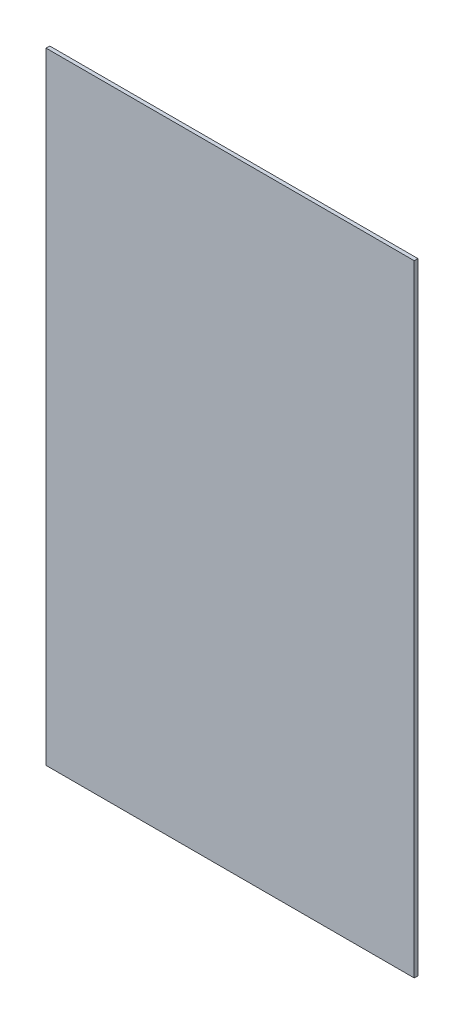
SolidWorks part; units mm, degrees
material "PMMA(有机玻璃)"
ref_plane "前视" through (0, 0, 0) normal (0, 0, 1) x (1, 0, 0)
ref_plane "上视" through (0, 0, 0) normal (0, 1, 0) x (1, 0, 0)
ref_plane "右视" through (0, 0, 0) normal (1, 0, 0) x (0, 0, -1)
sketch "草图1" plane through (0, 0, 0) normal (0, 0, 1) x (1, 0, 0)
  line L1 (-249.5, 421) -> (249.5, 421)
  line L2 (-249.5, 421) -> (-249.5, -421)
  line L3 (-249.5, -421) -> (249.5, -421)
  line L4 (249.5, 421) -> (249.5, -421)
  line L5 (-249.5, 421) -> (249.5, -421) construction
  line L6 (-249.5, -421) -> (249.5, 421) construction
  point P0 (0, 0)
  dimension "D1" = 842
  dimension "D2" = 499
extrude "凸台-拉伸1" add sketch "草图1" along normal blind 5
hole_wizard "M5 间隙孔1" positions "草图3" profile "草图2" hole size "M5" standard "GB"
sketch "草图3" plane through (0, 0, 5) normal (0, 0, 1) x (1, 0, 0)
  line L0 (-427.5, 273) -> (-427.5, -273) construction
  line L1 (-427.5, -273) -> (427.5, -273) construction
  line L2 (0, 273) -> (0, -273) construction
  line L3 (427.5, 273) -> (-427.5, 273) construction
  line L5 (-427.5, 0) -> (427.5, 0) construction
  line L6 (427.5, -273) -> (427.5, 273) construction
  point P0 (-375, -261)
  point P46 (415.5, 250)
  point P48 (-415.5, 250)
  point P58 (-125, -261)
  point P59 (125, -261)
  point P61 (-125, 261)
  point P62 (125, 261)
  point P64 (-375, 261)
  point P88 (375, -261)
  point P89 (375, 261)
  point P108 (415.5, 0)
  point P109 (-415.5, 0)
  point P110 (415.5, -250)
  point P111 (-415.5, -250)
  dimension "D1" = 12
  dimension "D2" = 12
  dimension "D5" = 3
  dimension "D3" = 12
  dimension "D6" = 4
  dimension "D4" = 2
sketch "草图2" plane through (-375, -261, 5) normal (1, 0, 0) x (0, -1, 0)
  line L0 (0, 0) -> (0, 5)
  line L1 (0, 5) -> (2.75, 5)
  line L2 (2.75, 5) -> (2.75, 0)
  line L5 (2.75, 0) -> (0, 0)
  line L11 (0, -6.35) -> (0, 107.95) construction
  dimension "通孔孔直径" = 5.5
  dimension "通孔孔深度" = 5
